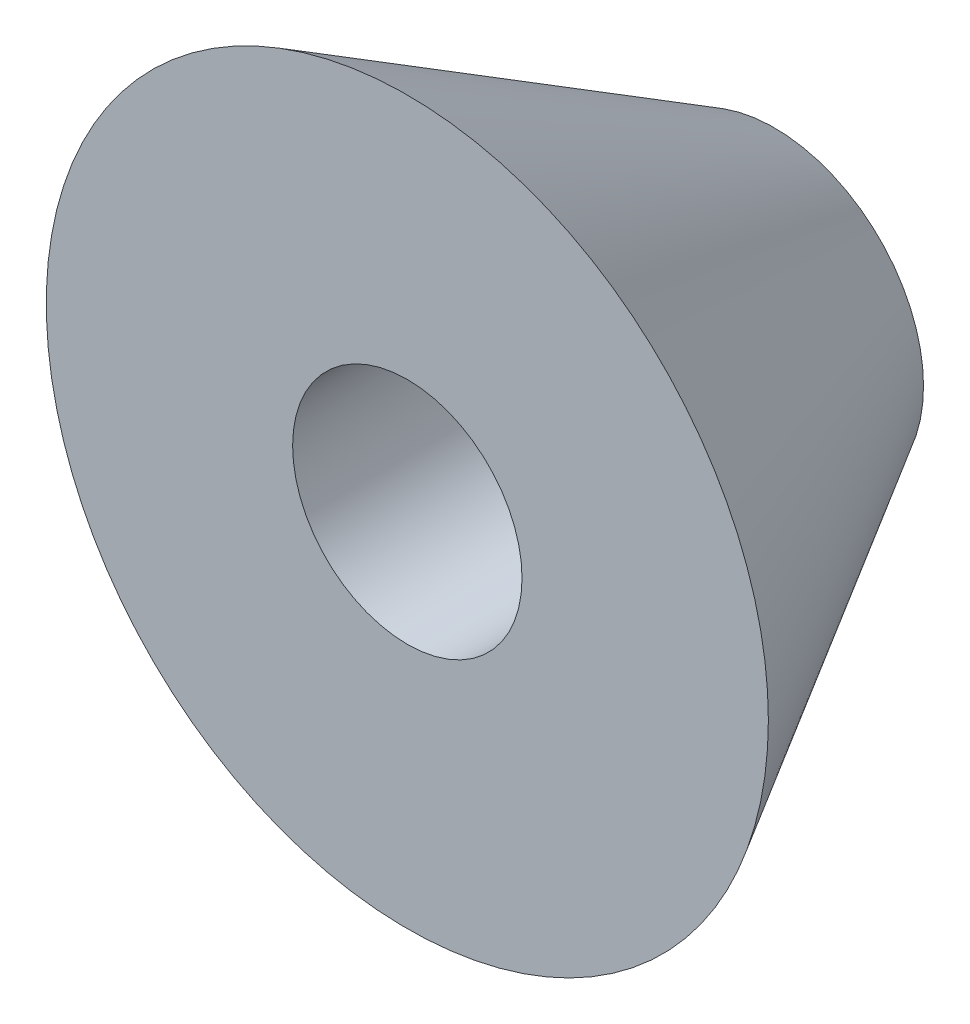
SolidWorks part; units mm, degrees
ref_plane "Front Plane" through (0, 0, 0) normal (0, 0, 1) x (1, 0, 0)
ref_plane "Top Plane" through (0, 0, 0) normal (0, 1, 0) x (1, 0, 0)
ref_plane "Right Plane" through (0, 0, 0) normal (1, 0, 0) x (0, 0, -1)
sketch "Sketch1" plane through (0, 0, 0) normal (0, 0, 1) x (1, 0, 0)
  circle A1 centre (0, 0) radius 3.25
  dimension "D2" = 6.5
extrude "Boss-Extrude1" add sketch "Sketch1" along normal blind 8 draft 30 draft outward yes
sketch "Sketch2" plane through (0, 0, 0) normal (0, 0, -1) x (-1, 0, 0)
  circle A0 centre (0, 0) radius 2.5
  dimension "D1" = 5
extrude "Cut-Extrude1" cut sketch "Sketch2" against normal through all
